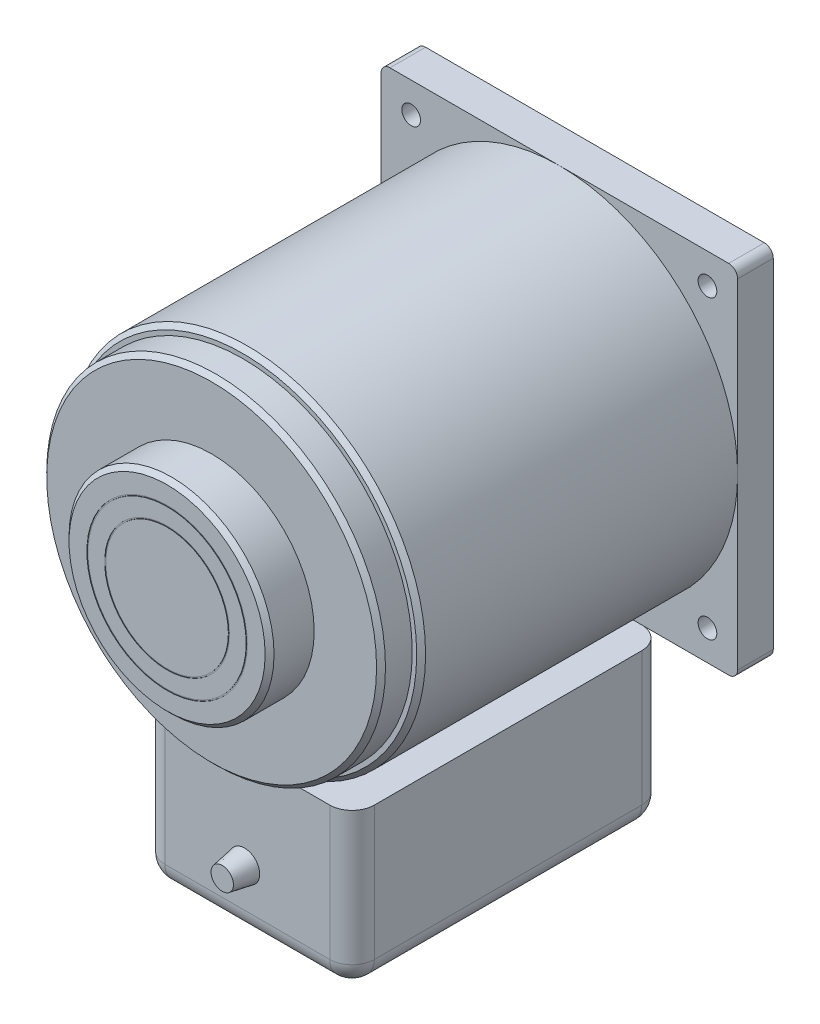
from build123d import *

# Parameters (mm, degrees)
SKETCH_1_W                  = 80
SKETCH_1_H                  = 80
EXTRUDE_1_DEPTH             = 8
SKETCH_2_R                  = 40
EXTRUDE_2_DEPTH             = 71
SKETCH_3_R                  = 38
EXTRUDE_3_DEPTH             = 7
SKETCH_4_R                  = 23
EXTRUDE_4_DEPTH             = 10
SKETCH_5_R                  = 4
EXTRUDE_5_DEPTH             = 20
FILLET_1_R                  = 2
CHAMFER_1_SIZE              = 1
SKETCH_6_R                  = 18
SKETCH_6_R_2                = 17.75
SKETCH_6_R_3                = 14
SKETCH_6_R_4                = 13.75
CUT_EXTRUDE_2_DEPTH         = 0.1
SKETCH_8_W                  = 47
SKETCH_8_H                  = 35
EXTRUDE_6_DEPTH             = 70
FILLET_2_R                  = 5
SKETCH_9_R                  = 3.398256342
EXTRUDE_7_DEPTH             = 5
EXTRUDE_7_TAPER             = 10
SKETCH_13_W                 = 2.1
SKETCH_13_H                 = 96
HOLE_WIZARD_M5_1_AT_2_COUNT = 2
HOLE_WIZARD_M5_1_AT_2_PITCH = 66.468037432
HOLE_WIZARD_M5_1_AT_3_COUNT = 2
HOLE_WIZARD_M5_1_AT_3_PITCH = 94
HOLE_WIZARD_M5_1_AT_4_COUNT = 2
HOLE_WIZARD_M5_1_AT_4_PITCH = 66.468037432


with BuildPart() as part:
    # 草图1 → 凸台-拉伸1 (new body)
    with BuildSketch(Plane.XY):
        with Locations((40, 40)):
            Rectangle(SKETCH_1_W, SKETCH_1_H)
    extrude(amount=EXTRUDE_1_DEPTH)

    # 草图2 → 凸台-拉伸2 (add)
    with BuildSketch(Plane.XY.offset(8)):
        with Locations((40, 40)):
            Circle(SKETCH_2_R)
    extrude(amount=EXTRUDE_2_DEPTH)

    # 草图3 → 凸台-拉伸3 (add)
    with BuildSketch(Plane.XY.offset(79)):
        with Locations((40, 40)):
            Circle(SKETCH_3_R)
    extrude(amount=EXTRUDE_3_DEPTH)

    # 草图4 → 凸台-拉伸4 (add)
    with BuildSketch(Plane.XY.offset(86)):
        with Locations((40, 40)):
            Circle(SKETCH_4_R)
    extrude(amount=EXTRUDE_4_DEPTH)

    # 草图5 → 凸台-拉伸5 (add)
    with BuildSketch(Plane(origin=(0, 0, 0), x_dir=(-1, 0, 0), z_dir=(0, 0, -1))):
        with Locations((-40, 40)):
            Circle(SKETCH_5_R)
    extrude(amount=EXTRUDE_5_DEPTH)

    # 圆角1
    fillet_1_edges = [part.edges().sort_by_distance(p)[0] for p in [
        (0, 80, 4),
        (80, 80, 4),
        (80, 0, 4),
        (0, 0, 4),
    ]]
    fillet(fillet_1_edges, radius=FILLET_1_R)

    # 倒角1
    chamfer_1_edges = [part.edges().sort_by_distance(p)[0] for p in [
        (0, 40, 79),
        (2, 40, 86),
        (17, 40, 96),
    ]]
    chamfer(chamfer_1_edges, length=CHAMFER_1_SIZE)

    # 草图6 → 切除-拉伸2 (cut)
    # profile 1 of 2: a face of its own
    with BuildSketch(Plane.XY.offset(96)):
        with Locations((40, 40)):
            Circle(SKETCH_6_R)
        with Locations((40, 40)):
            Circle(SKETCH_6_R_2, mode=Mode.SUBTRACT)
    # profile 2 of 2: a face of its own
    with BuildSketch(Plane.XY.offset(96)):
        with Locations((40, 40)):
            Circle(SKETCH_6_R_3)
        with Locations((40, 40)):
            Circle(SKETCH_6_R_4, mode=Mode.SUBTRACT)
    extrude(amount=-CUT_EXTRUDE_2_DEPTH, mode=Mode.SUBTRACT)

    # 草图13 → M5 螺纹孔1 (revolve, cut)
    with BuildSketch(Plane(origin=(73.234018716, 73.234018716, 0), x_dir=(0, 1, 0), z_dir=(1, 0, 0))):
        with Locations((1.05, 48)):
            Rectangle(SKETCH_13_W, SKETCH_13_H)
    hole_wizard_m5_1 = revolve(axis=Axis((73.234018716, 73.234018716, -6.35), (0, 0, 1)), mode=Mode.SUBTRACT)

    # M5 螺纹孔1 at 2: M5 螺纹孔1 ×2
    with Locations(*[(-i * HOLE_WIZARD_M5_1_AT_2_PITCH, 0, 0) for i in range(1, HOLE_WIZARD_M5_1_AT_2_COUNT)]):
        add(hole_wizard_m5_1, mode=Mode.SUBTRACT)

    # M5 螺纹孔1 at 3: M5 螺纹孔1 ×2
    with Locations(*[Vector(-0.7071067811865476, -0.7071067811865476, 0) * (i * HOLE_WIZARD_M5_1_AT_3_PITCH) for i in range(1, HOLE_WIZARD_M5_1_AT_3_COUNT)]):
        add(hole_wizard_m5_1, mode=Mode.SUBTRACT)

    # M5 螺纹孔1 at 4: M5 螺纹孔1 ×2
    with Locations(*[(0, -i * HOLE_WIZARD_M5_1_AT_4_PITCH, 0) for i in range(1, HOLE_WIZARD_M5_1_AT_4_COUNT)]):
        add(hole_wizard_m5_1, mode=Mode.SUBTRACT)


with BuildPart() as body_2:
    # 草图8 → 凸台-拉伸6 (new body)
    with BuildSketch(Plane.XY.offset(8)):
        with Locations((40, -17.5)):
            Rectangle(SKETCH_8_W, SKETCH_8_H)
    extrude(amount=EXTRUDE_6_DEPTH)

    # 圆角2
    fillet_2_edges = [body_2.edges().sort_by_distance(p)[0] for p in [
        (16.5, -17.5, 78),
        (40, -35, 78),
        (63.5, -17.5, 78),
        (40, -35, 8),
        (16.5, -17.5, 8),
        (63.5, -17.5, 8),
        (63.5, -35, 43),
        (16.5, -35, 43),
    ]]
    fillet(fillet_2_edges, radius=FILLET_2_R)

    # 草图9 → 凸台-拉伸7 (add)
    with BuildSketch(Plane.XY.offset(78)):
        with Locations((39.377618123, -21.300124573)):
            Circle(SKETCH_9_R)
    extrude(amount=EXTRUDE_7_DEPTH, taper=EXTRUDE_7_TAPER)


solid = Compound([part.part, body_2.part])
